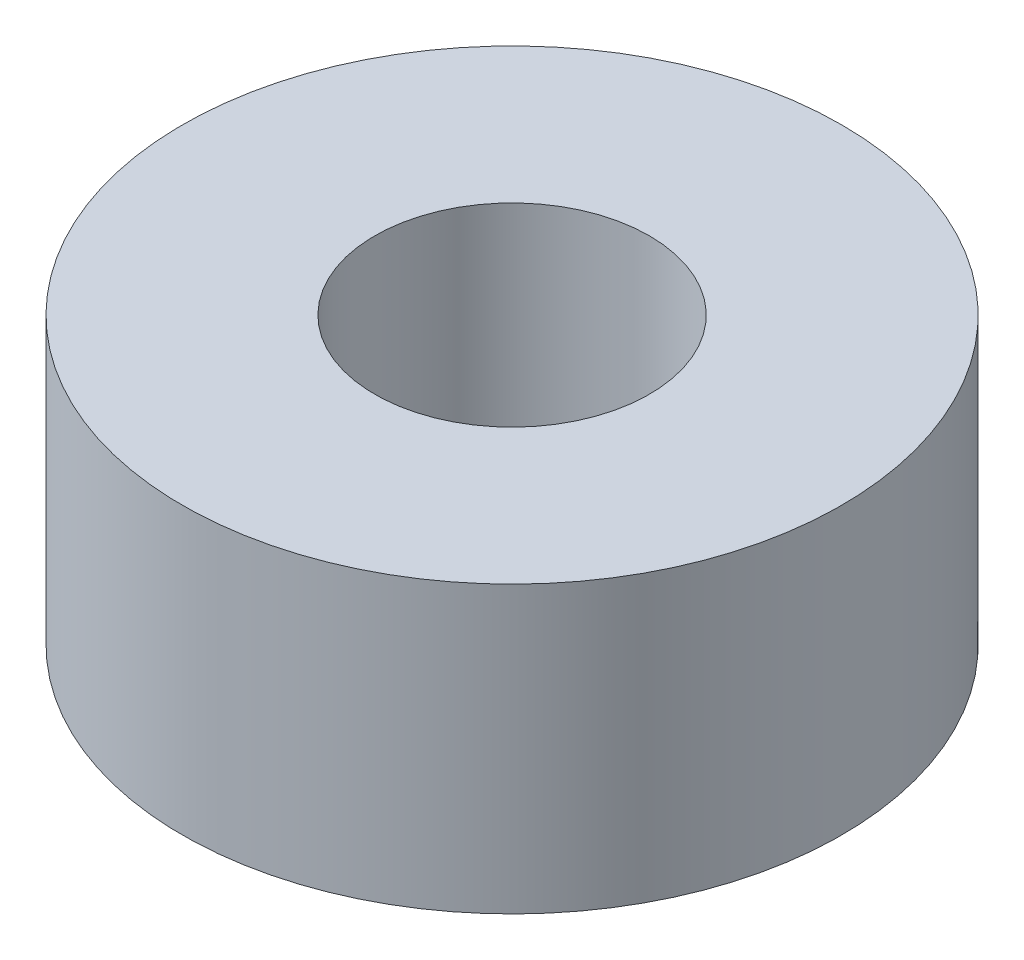
SolidWorks part; units mm, degrees
material "Q235B"
ref_plane "Front Plane" through (0, 0, 0) normal (0, 0, 1) x (1, 0, 0)
ref_plane "Top Plane" through (0, 0, 0) normal (0, 1, 0) x (1, 0, 0)
ref_plane "Right Plane" through (0, 0, 0) normal (1, 0, 0) x (0, 0, -1)
sketch "Sketch1" plane through (0, 0, 0) normal (0, 0, 1) x (1, 0, 0)
  line L0 (25, 0) -> (25, 60)
  line L1 (25, 60) -> (60, 60)
  line L2 (60, 60) -> (60, 8)
  line L3 (60, 8) -> (35, 8)
  line L4 (35, 8) -> (35, 0)
  line L5 (35, 0) -> (25, 0)
  line L6 (0, 0) -> (0, 51.1204) construction
  dimension "D1" = 70
  dimension "D2" = 120
  dimension "D3" = 50
  dimension "D4" = 60
  dimension "D5" = 52
revolve "Revolve1" add sketch "Sketch1" angle 360 about L6
